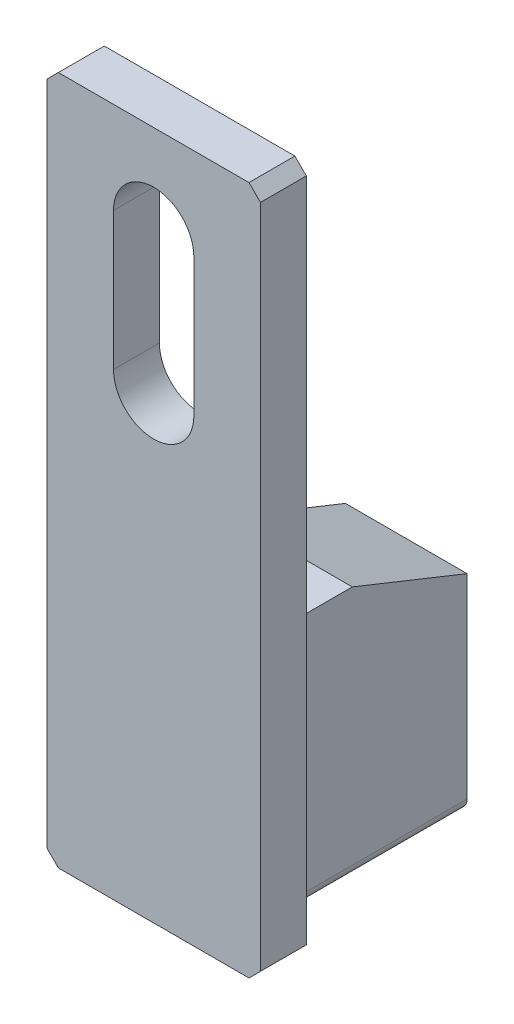
from build123d import *

# Parameters (mm, degrees)
SKETCH1_W           = 5.3
SKETCH1_H           = 11
BOSS_EXTRUDE1_DEPTH = 9
SKETCH2_W           = 9.3
SKETCH2_H           = 30
BOSS_EXTRUDE2_DEPTH = 2
CUT_EXTRUDE1_DEPTH  = 10
CHAMFER1_SIZE       = 0.5
FILLET1_R           = 0.5
CHAMFER2_SIZE       = 2
CHAMFER2_SIZE2      = 5


with BuildPart() as part:
    # Sketch1 → Boss-Extrude1 (new body)
    with BuildSketch(Plane.XY):
        Rectangle(SKETCH1_W, SKETCH1_H)
    extrude(amount=BOSS_EXTRUDE1_DEPTH)

    # Sketch2 → Boss-Extrude2 (add)
    with BuildSketch(Plane.XY.offset(9)):
        with Locations((0, 9.5)):
            Rectangle(SKETCH2_W, SKETCH2_H)
    extrude(amount=BOSS_EXTRUDE2_DEPTH)

    # Sketch3 → Cut-Extrude1 (cut)
    with BuildSketch(Plane.XY.offset(11)):
        with BuildLine():
            Line((1.75, 20.5), (1.75, 14.5))
            ThreePointArc((1.75, 14.5), (0, 12.75), (-1.75, 14.5))
            Line((-1.75, 14.5), (-1.75, 20.5))
            ThreePointArc((-1.75, 20.5), (0, 22.25), (1.75, 20.5))
        make_face()
    extrude(amount=-CUT_EXTRUDE1_DEPTH, mode=Mode.SUBTRACT)

    # Chamfer1
    chamfer1_edges = [part.edges().sort_by_distance(p)[0] for p in [
        (-4.65, -5.5, 10),
        (4.65, -5.5, 10),
        (4.65, 24.5, 10),
        (-4.65, 24.5, 10),
    ]]
    chamfer(chamfer1_edges, length=CHAMFER1_SIZE)

    # Fillet1
    fillet1_edges = [part.edges().sort_by_distance(p)[0] for p in [
        (2.65, -5.5, 4.5),
        (-2.65, -5.5, 4.5),
    ]]
    fillet(fillet1_edges, radius=FILLET1_R)

    # Chamfer2
    chamfer2_edges = [part.edges().sort_by_distance(p)[0] for p in [
        (0, 5.5, 0),
    ]]
    chamfer2_side = [part.faces().sort_by_distance(p)[0] for p in [
        (0, 0.00993546, 0),
    ]]
    chamfer(chamfer2_edges, length=CHAMFER2_SIZE, length2=CHAMFER2_SIZE2, reference=chamfer2_side[0])


solid = part.part
